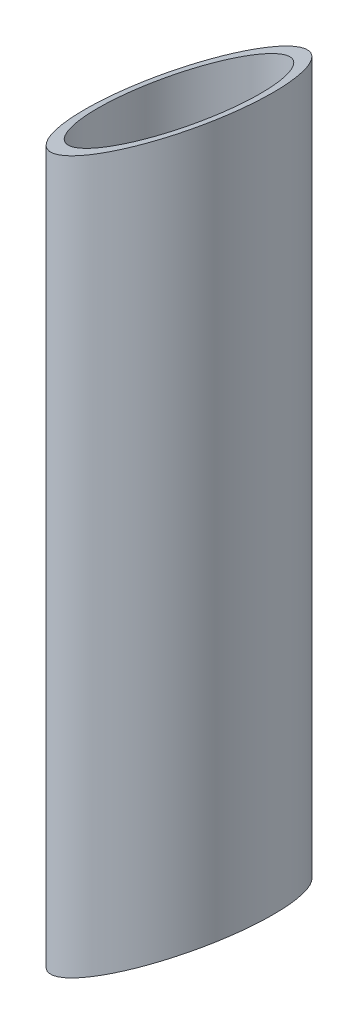
from build123d import *

# Parameters (mm, degrees)
SKETCH1_R               = 11
SKETCH1_R_2             = 9.5
BOSS_EXTRUDE1_DEPTH     = 48
CUT_EXTRUDE1_DEPTH      = 51.457903246
CUT_EXTRUDE1_DEPTH_BACK = 51.457903246


with BuildPart() as part:
    # Sketch1 → Boss-Extrude1 (new, symmetric)
    with BuildSketch(Plane(origin=(0, 0, 0), x_dir=(1, 0, 0), z_dir=(0, 1, 0))):
        with Locations(Location((0, 0, 0), (0, 0, 270))):
            Circle(SKETCH1_R)
        with Locations(Location((0, 0, 0), (0, 0, 270))):
            Circle(SKETCH1_R_2, mode=Mode.SUBTRACT)
    extrude(amount=BOSS_EXTRUDE1_DEPTH, both=True)

    # Sketch2 → Cut-Extrude1 (cut, two sides: drawn at the far end of the back side and taken through both)
    with BuildSketch(Plane.XY.offset(-CUT_EXTRUDE1_DEPTH_BACK)):
        Polygon((11, 48), (-11, 48), (-11, 35.298294078), align=None)
        Polygon((11, -35.298294078), (11, -48), (-11, -48), align=None)
    extrude(amount=CUT_EXTRUDE1_DEPTH + CUT_EXTRUDE1_DEPTH_BACK, mode=Mode.SUBTRACT)


solid = part.part
